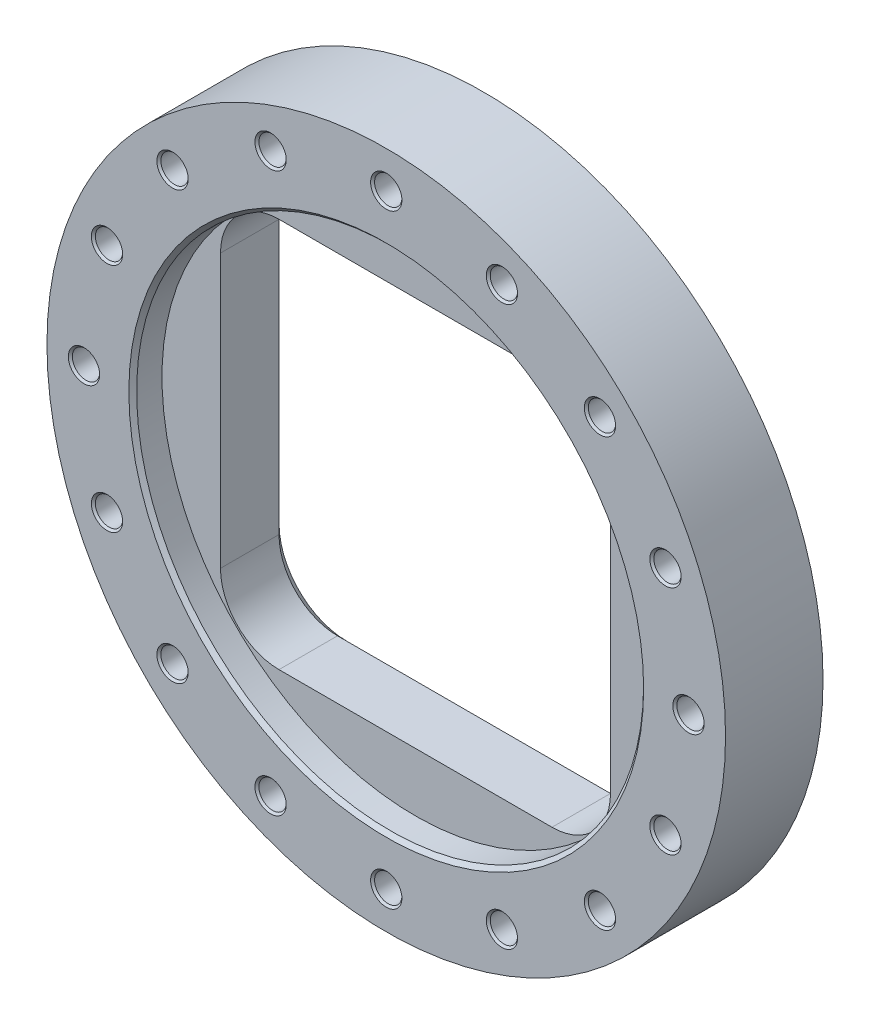
SolidWorks part; units mm, degrees
material "Q345"
ref_plane "前视基准面" through (0, 0, 0) normal (0, 0, 1) x (1, 0, 0)
ref_plane "上视基准面" through (0, 0, 0) normal (0, 1, 0) x (1, 0, 0)
ref_plane "右视基准面" through (0, 0, 0) normal (1, 0, 0) x (0, 0, -1)
sketch "草图1" plane through (0, 0, 0) normal (0, 0, 1) x (1, 0, 0)
  line L1 (-90, 90) -> (90, 90) construction
  line L2 (-90, 90) -> (-90, -90) construction
  line L3 (-90, -90) -> (90, -90) construction
  line L4 (90, 90) -> (90, -90) construction
  line L5 (-90, 90) -> (90, -90) construction
  line L6 (-90, -90) -> (90, 90) construction
  circle A0 centre (0, 0) radius 174
  dimension "D1" = 348
  dimension "D2" = 180
  dimension "D3" = 180
extrude "凸台-拉伸1" add sketch "草图1" along normal blind 50
sketch "草图2" plane through (0, 0, 50) normal (0, 0, 1) x (1, 0, 0)
  line L1 (-70, 100) -> (70, 100)
  line L2 (-100, 70) -> (-100, -70)
  line L3 (-70, -100) -> (70, -100)
  line L4 (100, 70) -> (100, -70)
  line L5 (-100, 100) -> (100, -100) construction
  line L6 (-100, -100) -> (100, 100) construction
  arc A0 (-70, -100) -> (-100, -70) centre (-70, -70) cw
  arc A1 (70, -100) -> (100, -70) centre (70, -70) ccw
  arc A2 (100, 70) -> (70, 100) centre (70, 70) ccw
  arc A3 (-100, 70) -> (-70, 100) centre (-70, 70) cw
  point P0 (0, 0)
  dimension "D3" = 30
  dimension "D1" = 200
  dimension "D2" = 200
extrude "切除-拉伸1" cut sketch "草图2" against normal through all
sketch "草图3" plane through (0, 0, 50) normal (0, 0, 1) x (1, 0, 0)
  circle A0 centre (0, 0) radius 155
  circle A1 centre (0, 155) radius 10
  dimension "D1" = 310
  dimension "D2" = 20
hole_wizard "M16 螺纹孔1" positions "3D草图1" profile "草图4" tap size "M16" standard "GB" end condition up to next
sketch3d "3D草图1"
  point P0 (0, 155, 50)
sketch "草图4" plane through (0, 155, 50) normal (1, 0, 0) x (0, -1, 0)
  line L0 (0, 0) -> (0, 50)
  line L1 (0, 50) -> (7, 50)
  line L2 (7, 50) -> (7, 1.025)
  line L3 (7, 1.025) -> (8.025, 0)
  line L5 (8.025, 0) -> (0, 0)
  line L6 (-7, 1.025) -> (-8.025, 0) construction
  line L11 (0, -6.35) -> (0, 107.95) construction
  dimension "通孔螺纹孔钻头直径" = 14
  dimension "通孔螺纹孔钻头深度" = 50
  dimension "近端锥形沉头孔直径" = 16.05
  dimension "近端锥形沉头孔角度" = 90
cosmetic thread "孔螺蚊线1" parameters "D2"=16
pattern_circular "阵列(圆周)1" count 16 over 360 about axis through (0, 0, 0) along (0, 0, 1) of "M16 螺纹孔1"
sketch "草图5" plane through (0, 0, 50) normal (0, 0, 1) x (1, 0, 0)
  line L0 (0, 174) -> (0, -174) construction
  circle A0 centre (0, 0) radius 174 construction
  circle A1 centre (0, 0) radius 130
  dimension "D1" = 260
extrude "切除-拉伸2" cut sketch "草图5" against normal blind 15
chamfer "倒角1" distance 2 angle 45 1 edges at (130, 0, 50)
chamfer "倒角2" distance 5 angle 45 8 edges at (-91.2132, -91.2132, 0) (0, -100, 0) (-100, 0, 0) (91.2132, -91.2132, 0) (-91.2132, 91.2132, 0) (100, 0, 0) (91.2132, 91.2132, 0) (0, 100, 0)
